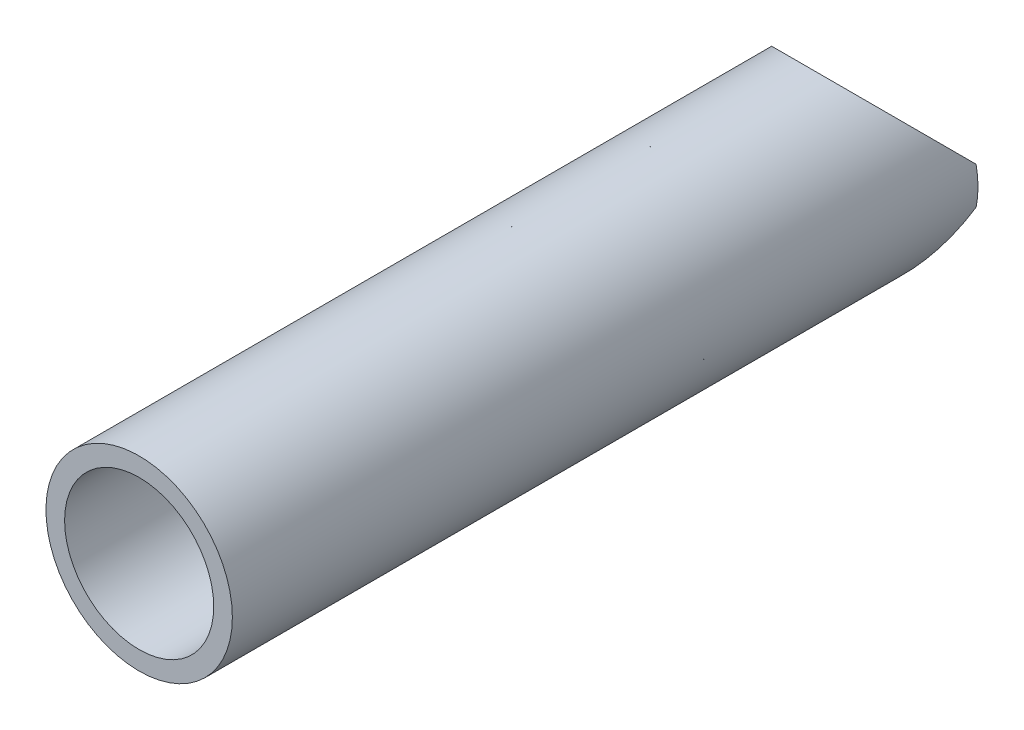
from build123d import *

# Parameters (mm, degrees)
SKETCH_1_R               = 25
SKETCH_1_R_2             = 20
EXTRUDE_1_DEPTH          = 200
CUT_EXTRUDE_1_DEPTH      = 500
CUT_EXTRUDE_1_DEPTH_BACK = 204.100960116
SKETCH_2_R               = 25


with BuildPart() as part:
    # 草图1 → 凸台-拉伸1 (new body)
    with BuildSketch(Plane.XY):
        Circle(SKETCH_1_R)
        Circle(SKETCH_1_R_2, mode=Mode.SUBTRACT)
    extrude(amount=EXTRUDE_1_DEPTH)

    # 草图2 → 切除-拉伸1 (cut, two sides: drawn at the far end of the back side and taken through both)
    with BuildSketch(Plane(origin=(0, 0, 0), x_dir=(1, 0, 0), z_dir=(0, 1, 0)).offset(-CUT_EXTRUDE_1_DEPTH_BACK)):
        with Locations((0, 5)):
            Circle(SKETCH_2_R)
    extrude(amount=CUT_EXTRUDE_1_DEPTH + CUT_EXTRUDE_1_DEPTH_BACK, mode=Mode.SUBTRACT)


solid = part.part
